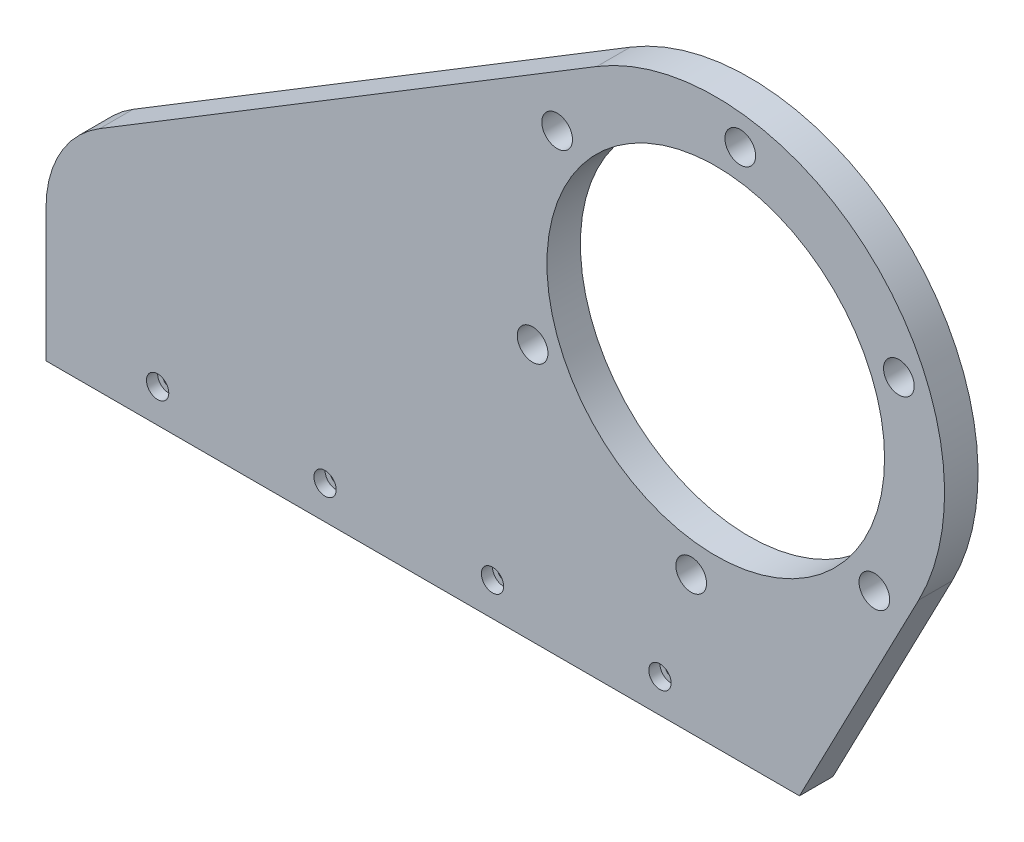
from build123d import *

# Parameters (mm, degrees)
EXTRUDE_1_DEPTH     = 12
SKETCH_2_R          = 60.5
CUT_EXTRUDE_2_DEPTH = 269.596351427
SKETCH_3_R          = 2
CUT_EXTRUDE_3_DEPTH = 269.596351427
SKETCH_4_R          = 4
CUT_EXTRUDE_4_DEPTH = 4
CUT_EXTRUDE_START   = -4
SKETCH_5_R          = 4
CUT_EXTRUDE_5_DEPTH = 4
SKETCH_6_R          = 5.5
CUT_EXTRUDE_6_DEPTH = 269.596351427


with BuildPart() as part:
    # 草图1 → 凸台-拉伸1 (new body)
    with BuildSketch(Plane.XY):
        with BuildLine():
            Line((0, -120), (-240, -120))
            Line((-240, -120), (-240, -72.488505))
            ThreePointArc((-240, -72.488505), (-234.867302193, -52.885667507), (-220.786438112, -38.313602065))
            Line((-220.786438112, -38.313602065), (-42.612198129, 70.058551017))
            ThreePointArc((-42.612198129, 70.058551017), (56.016961424, 59.884054913), (72.743129476, -37.847550964))
            Line((72.743129476, -37.847550964), (30, -120))
            Line((30, -120), (0, -120))
        make_face()
    extrude(amount=EXTRUDE_1_DEPTH)

    # 草图2 → 切除-拉伸2 (cut, through all)
    with BuildSketch(Plane.XY):
        Circle(SKETCH_2_R)
    extrude(amount=CUT_EXTRUDE_2_DEPTH, mode=Mode.SUBTRACT)

    # 草图3 → 切除-拉伸3 (cut, through all)
    with BuildSketch(Plane.XY.offset(12)):
        with Locations((-200, -108)):
            Circle(SKETCH_3_R)
        with Locations((-140, -108)):
            Circle(SKETCH_3_R)
        with Locations((-80, -108)):
            Circle(SKETCH_3_R)
        with Locations((-20, -108)):
            Circle(SKETCH_3_R)
    extrude(amount=-CUT_EXTRUDE_3_DEPTH, mode=Mode.SUBTRACT)

    # 草图4 → 切除-拉伸4 (cut)
    with BuildSketch(Plane.XY.offset(12)):
        with Locations((-200, -108)):
            Circle(SKETCH_4_R)
        with Locations((-140, -108)):
            Circle(SKETCH_4_R)
        with Locations((-80, -108)):
            Circle(SKETCH_4_R)
        with Locations((-20, -108)):
            Circle(SKETCH_4_R)
    extrude(amount=-CUT_EXTRUDE_4_DEPTH, mode=Mode.SUBTRACT)

    # 草图5 → 切除-拉伸5 (cut)
    with BuildSketch(Plane(origin=(0, 0, 0), x_dir=(-1, 0, 0), z_dir=(0, 0, -1)).offset(CUT_EXTRUDE_START)):
        with Locations(Location((20, -108, 0), (0, 0, 180))):
            Circle(SKETCH_5_R)
        with Locations(Location((80, -108, 0), (0, 0, 180))):
            Circle(SKETCH_5_R)
        with Locations(Location((140, -108, 0), (0, 0, 180))):
            Circle(SKETCH_5_R)
        with Locations(Location((200, -108, 0), (0, 0, 180))):
            Circle(SKETCH_5_R)
    extrude(amount=CUT_EXTRUDE_5_DEPTH, mode=Mode.SUBTRACT)

    # 草图6 → 切除-拉伸6 (cut, through all)
    with BuildSketch(Plane(origin=(0, 0, 0), x_dir=(-1, 0, 0), z_dir=(0, 0, -1))):
        with Locations((56.836099532, 42.967665634)):
            Circle(SKETCH_6_R)
        with Locations((-8.793040215, 70.705338863)):
            Circle(SKETCH_6_R)
        with Locations((65.629139746, -27.737673229)):
            Circle(SKETCH_6_R)
        with Locations((8.793040215, -70.705338863)):
            Circle(SKETCH_6_R)
        with Locations((-56.836099532, -42.967665634)):
            Circle(SKETCH_6_R)
        with Locations((-65.629139746, 27.737673229)):
            Circle(SKETCH_6_R)
    extrude(amount=-CUT_EXTRUDE_6_DEPTH, mode=Mode.SUBTRACT)


solid = part.part
